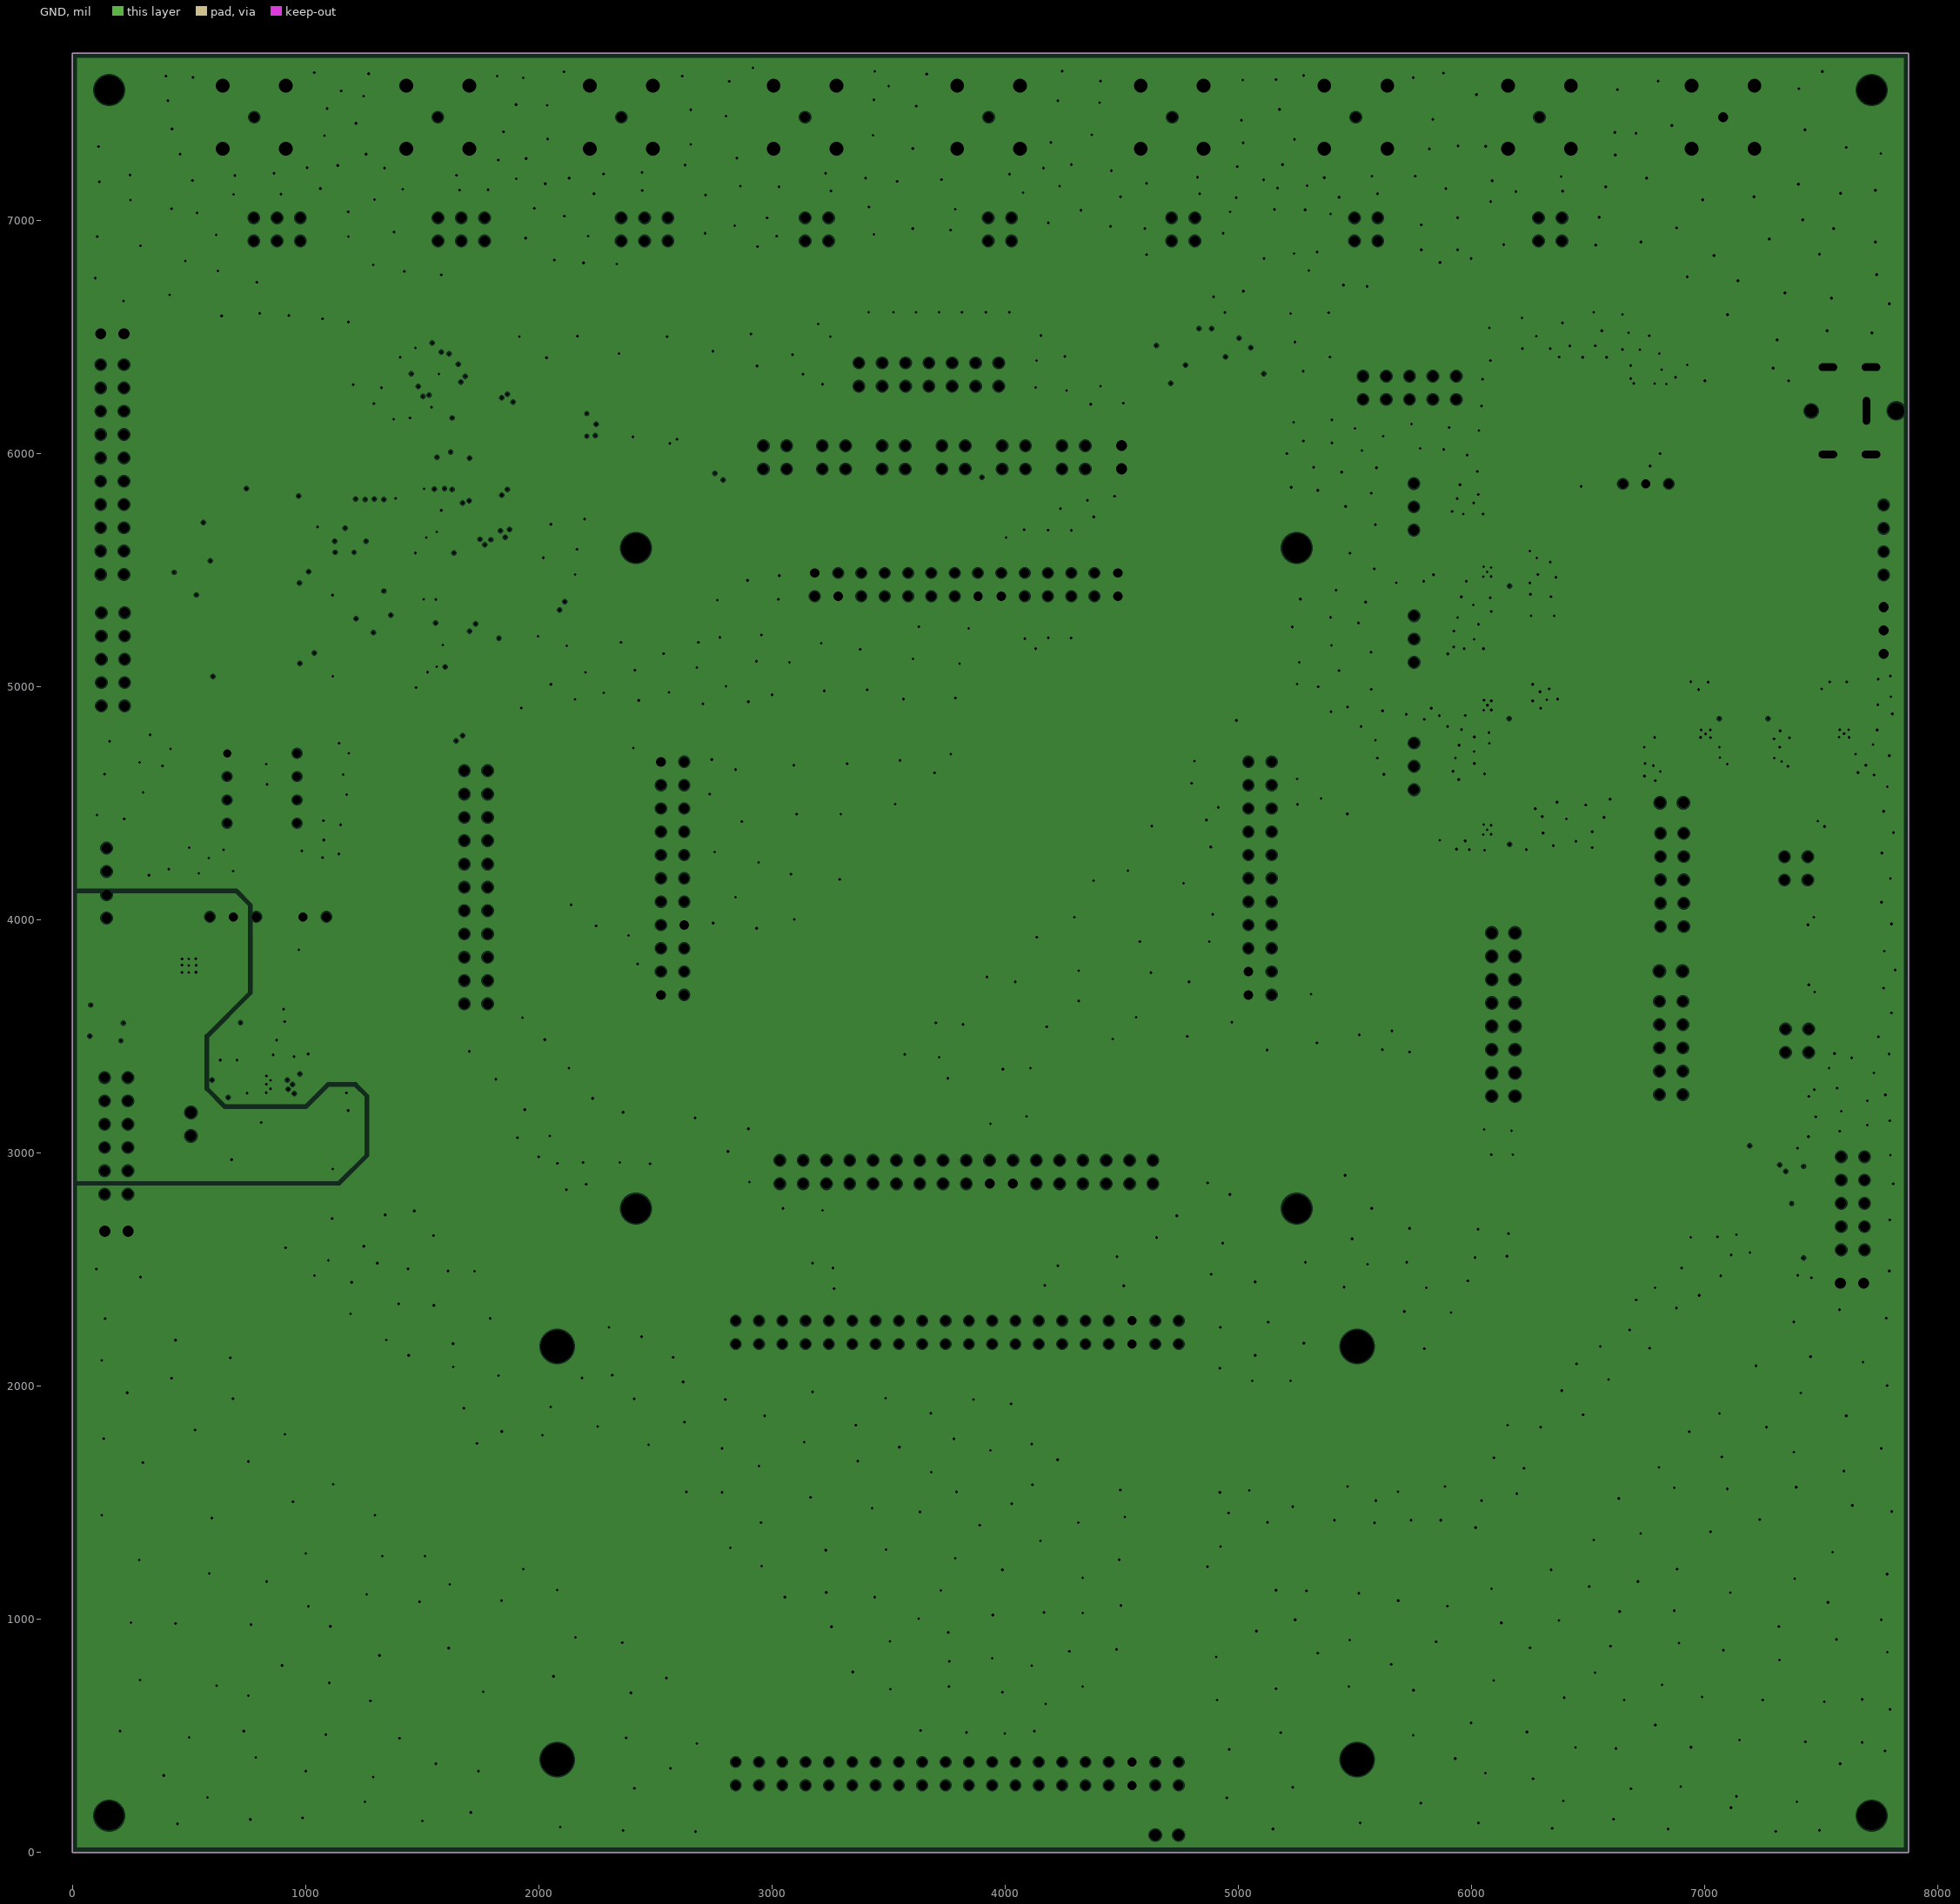
[diagram p0: GND, clearances drawn from the general rule]
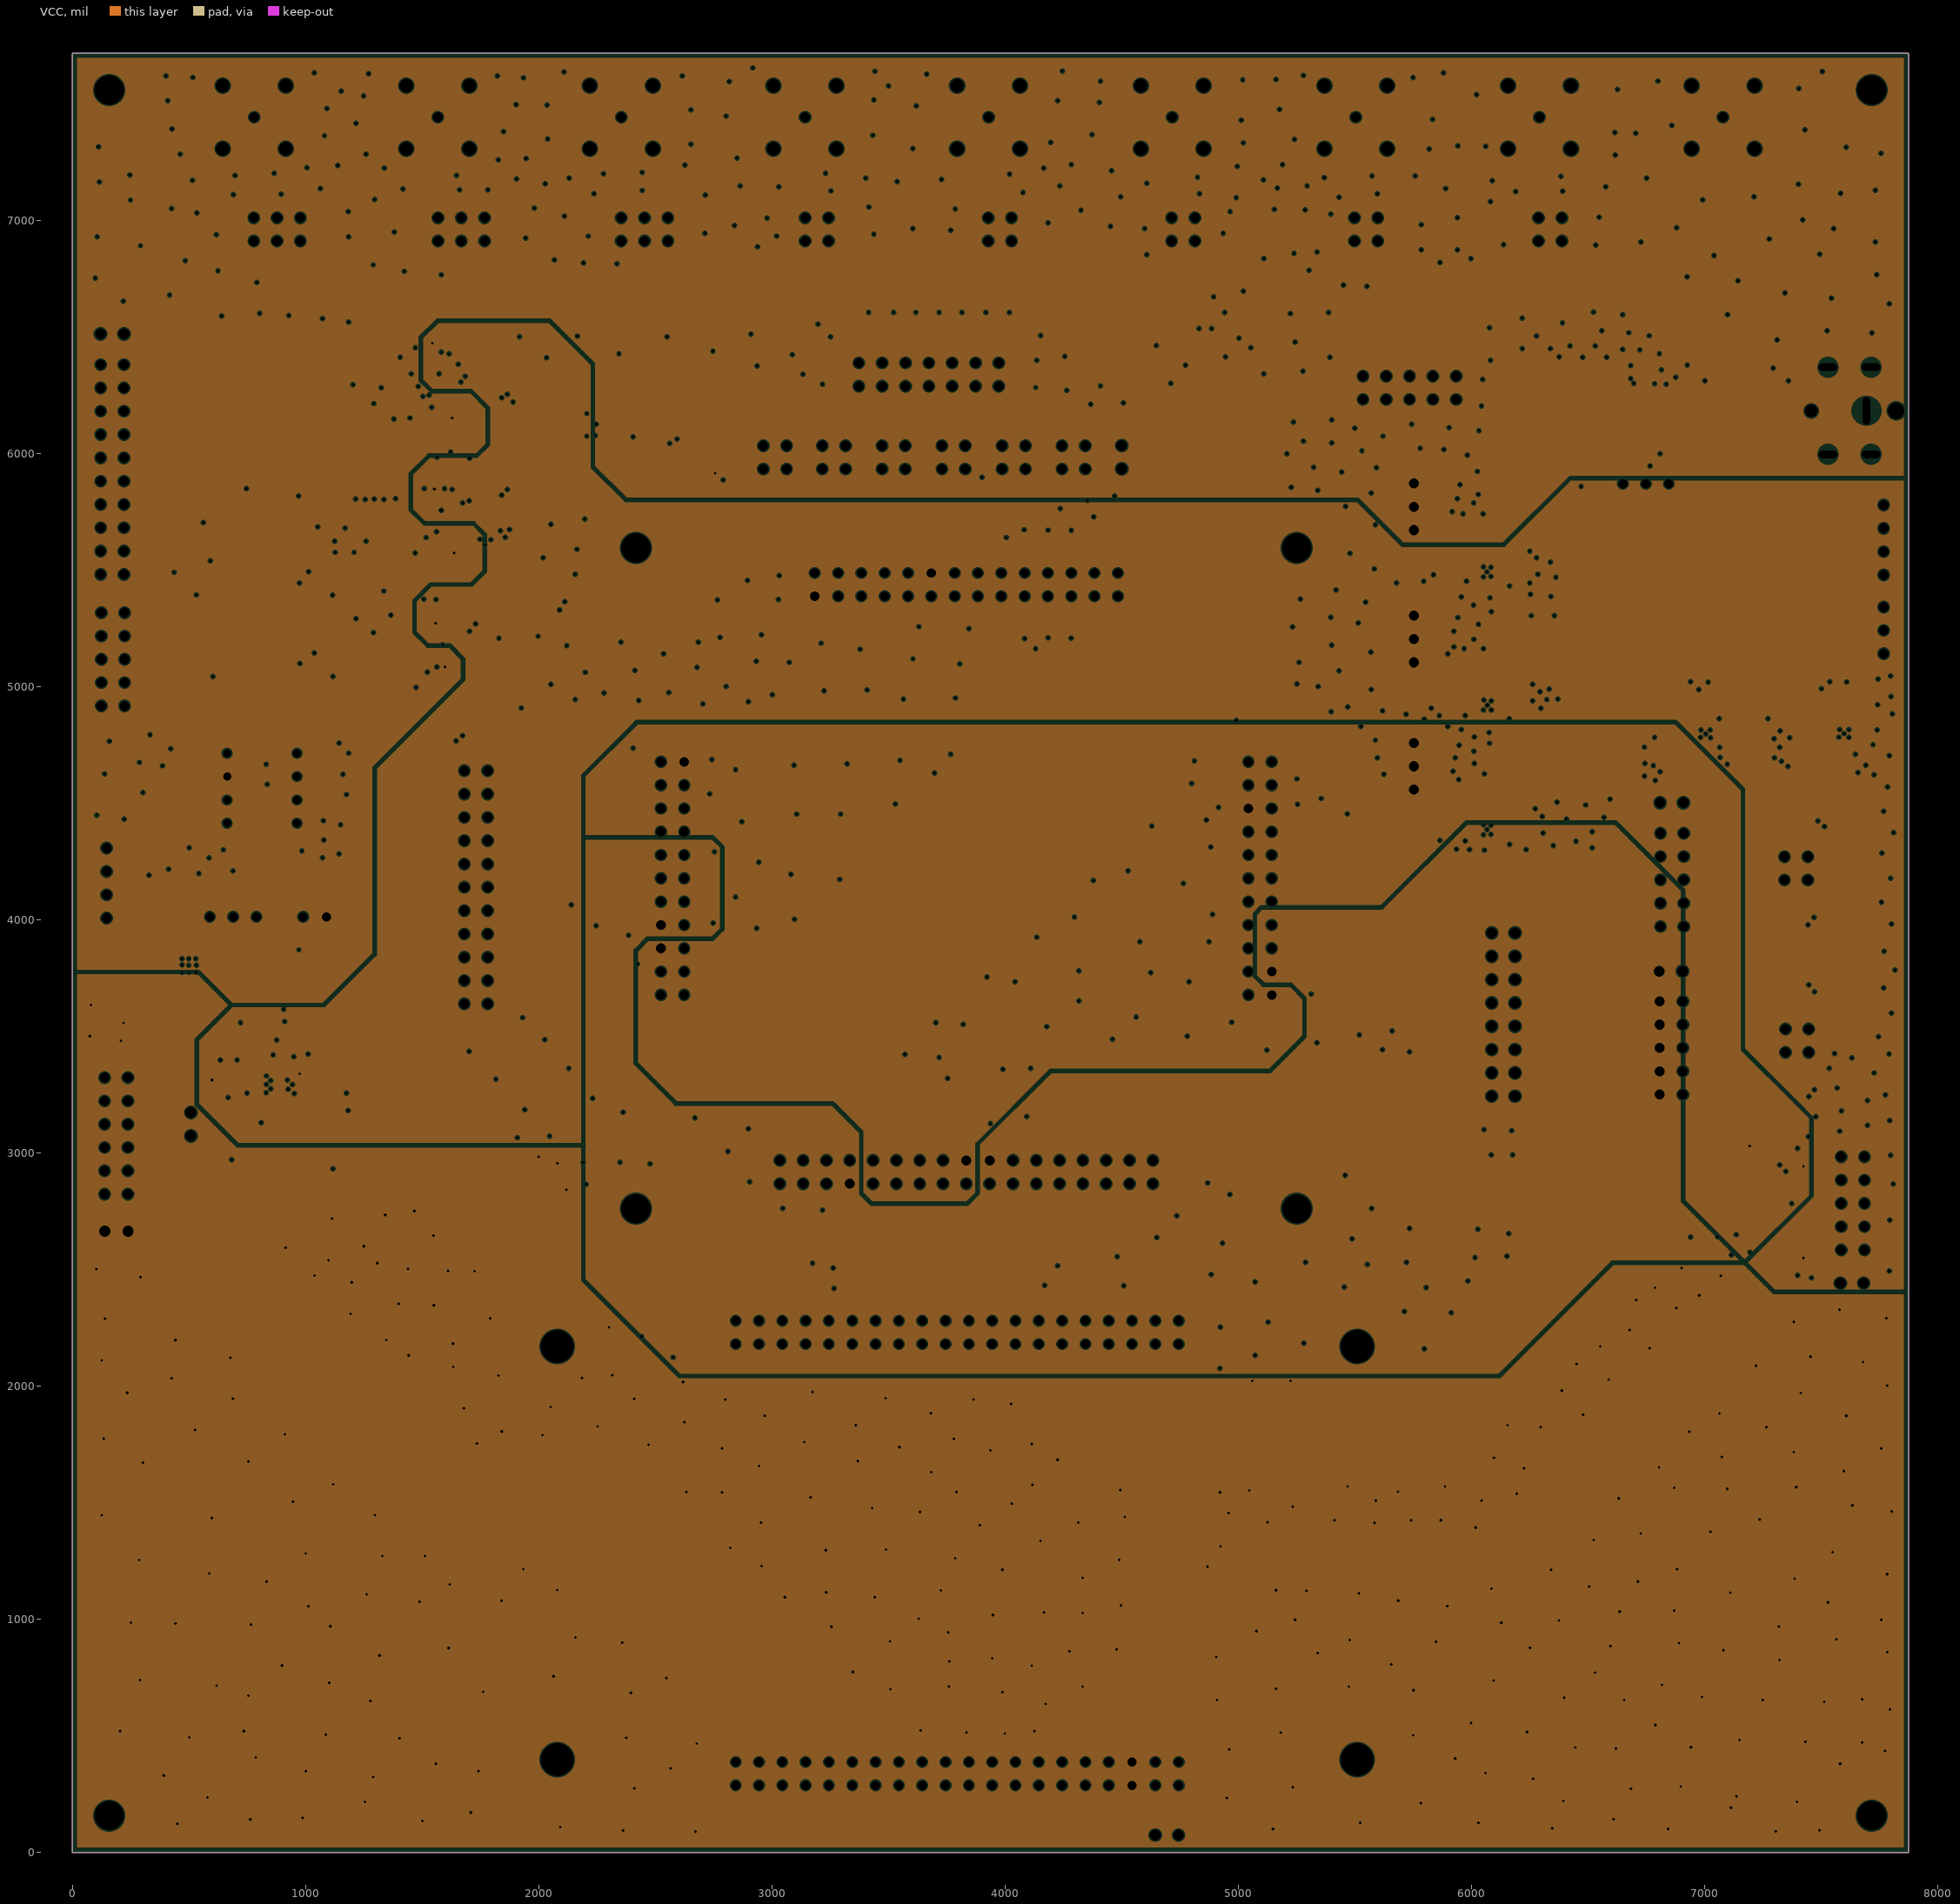
[diagram p1: VCC, clearances drawn from the general rule]
# Altium PCB MISC62793.pcbdoc (part 2 of 6)
## Footprints (in the part's own frame and the unit in brackets; to place one, negate y for a bottom-side part, rotate by r counter-clockwise, add the part's x,y. Pads: shape width x height; smd on the part's side, far side on the other; paste and mask are expansions set on the pad) (continued)
C0402 [mm]
  rect 0.79x0.54 smd paste-100 mask+0.051: 1(-0.545,0) 2(0.545,0)
  silkscreen extent -1.17,-0.5 1.17,0.5
C0603 [mm]
  rect 0.8x0.9 smd: 1(-0.7,0) 2(0.7,0)
  silkscreen extent -1.41,-0.71 1.39,0.72
C0805 [mm]
  rect 1.41x1.35 smd paste-100 mask+0.051: 1(-1,0) 2(1,0)
  silkscreen extent -1.96,-0.9 1.96,0.9
C1206 [mm]
  rect 1.485x1.728 smd paste-100 mask+0.051: 1(-1.593,0) 2(1.593,0)
  silkscreen extent -2.56,-1.09 2.56,1.09
C1210 [mm]
  rect 1.635x2.7 smd paste-100 mask+0.051: 1(-1.517,0) 2(1.517,0)
  silkscreen extent -2.56,-1.58 2.56,1.58
DC-IN-TH_HX-DC007B-2.5 [mm]
  round 1.8 hole 1.8 unplated: 0(-6,0)
  round 2.2 hole 1.4: 1(3.25,0)
  oval 1.4x3.8 hole 0.8 slot 3 at 90 deg: 2(-2.75,0)
  oval 2.8x1.4 hole 0.8 slot 2 at 0 deg: 3(-3.25,4.75) 3(-3.25,-4.75) 3(1.45,4.75) 3(1.45,-4.75)
  silkscreen extent -8.75,-5 4.25,5
DIP-8_L10.1-W6.3-P2.54-LS7.6-BL [mm]
  rect 1.5x1.5 hole 0.9: 1(-3.81,-3.81)
  round 1.5 hole 0.9: 2(-1.27,-3.81) 3(1.27,-3.81) 4(3.81,-3.81) 5(3.81,3.81) 6(1.27,3.81) 7(-1.27,3.81) 8(-3.81,3.81)
  silkscreen extent -5.23,-3.93 5.01,3.18
FILTER-SMD_4P-L7.0-W6.0-TL_SMCM7060 [mm]
  rect 2.5x1.75 smd: 1(-2.75,1.625) 2(-2.75,-1.625) 3(2.75,-1.625) 4(2.75,1.625)
  silkscreen extent -3.94,-3.05 3.94,3.05
HDR-TH_2P-P2.54-V-M [mm]
  rect 2x2 hole 1.2: 1(-1.27,0)
  round 2 hole 1.2: 2(1.27,0)
  silkscreen extent -2.54,-1.27 2.54,1.27
HDR-TH_3P-P2.54-V-M [mm]
  rect 1.7x1.7 hole 1.1: 1(-2.54,0)
  round 1.7 hole 1.1: 2(0,0) 3(2.54,0)
  silkscreen extent -4.02,-1.27 4.02,1.27
HDR-TH_4P-P2.54-V-M [mm]
  rect 1.7x1.7 hole 1.1: 1(-3.81,0)
  round 1.7 hole 1.1: 2(-1.27,0) 3(1.27,0) 4(3.81,0)
  silkscreen extent -5.08,-1.27 5.08,1.27
HDR-TH_4P-P2.54-V-M-R2-C2-S2.54 [mm]
  rect 1.7x1.7 hole 1.1: 1(-1.27,-1.27)
  round 1.7 hole 1.1: 2(-1.27,1.27) 3(1.27,-1.27) 4(1.27,1.27)
  silkscreen extent -2.77,-2.54 2.77,2.54
HDR-TH_6P-P2.54-V-M-R2-C3-S2.54 [mm]
  rect 1.7x1.7 hole 1.1: 1(-2.54,-1.27)
  round 1.7 hole 1.1: 2(-2.54,1.27) 3(0,-1.27) 4(0,1.27) 5(2.54,-1.27) 6(2.54,1.27)
  silkscreen extent -4.04,-2.54 4.04,2.54
HDR-TH_10P-P2.54-V-M-R2-C5-S2.54 [mm]
  rect 1.7x1.7 hole 1.1: 1(-5.08,-1.27)
  round 1.7 hole 1.1: 2(-5.08,1.27) 3(-2.54,-1.27) 4(-2.54,1.27) 5(0,-1.27) 6(0,1.27) 7(2.54,-1.27) 8(2.54,1.27) 9(5.08,-1.27) 10(5.08,1.27)
  silkscreen extent -6.35,-2.54 6.35,2.54
HDR-TH_12P-P2.54-V-M-R2-C6-S2.54 [mm]
  rect 1.7x1.7 hole 1.1: 1(-6.35,-1.27)
  round 1.7 hole 1.1: 2(-6.35,1.27) 3(-3.81,-1.27) 4(-3.81,1.27) 5(-1.27,-1.27) 6(-1.27,1.27) 7(1.27,-1.27) 8(1.27,1.27) 9(3.81,-1.27) 10(3.81,1.27) 11(6.35,-1.27) 12(6.35,1.27)
  silkscreen extent -7.85,-2.54 7.85,2.54
HDR-TH_14P-P2.54-V-M-R2-C7-S2.54 [mm]
  rect 1.7x1.7 hole 1.1: 1(-7.62,-1.27)
  round 1.7 hole 1.1: 2(-7.62,1.27) 3(-5.08,-1.27) 4(-5.08,1.27) 5(-2.54,-1.27) 6(-2.54,1.27) 7(0,-1.27) 8(0,1.27) 9(2.54,-1.27) 10(2.54,1.27) 11(5.08,-1.27) 12(5.08,1.27) 13(7.62,-1.27) 14(7.62,1.27)
  silkscreen extent -9.12,-2.54 9.12,2.54
HDR-TH_16P-P2.54-V-M-R2-C8-S2.54 [mm]
  rect 1.8x1.8 hole 1.2: 1(-8.89,-1.27)
  round 1.8 hole 1.2: 2(-8.89,1.27) 3(-6.35,-1.27) 4(-6.35,1.27) 5(-3.81,-1.27) 6(-3.81,1.27) 7(-1.27,-1.27) 8(-1.27,1.27) 9(1.27,-1.27) 10(1.27,1.27) 11(3.81,-1.27) 12(3.81,1.27) 13(6.35,-1.27) 14(6.35,1.27) 15(8.89,-1.27) 16(8.89,1.27)
  silkscreen extent -10.16,-2.54 10.16,2.54
HDR-TH_20P-P2.54-V-M-R2-C10-S2.54 [mm]
  rect 1.7x1.7 hole 1.1: 1(-11.43,-1.27)
  round 1.7 hole 1.1: 2(-11.43,1.27) 3(-8.89,-1.27) 4(-8.89,1.27) 5(-6.35,-1.27) 6(-6.35,1.27) 7(-3.81,-1.27) 8(-3.81,1.27) 9(-1.27,-1.27) 10(-1.27,1.27) 11(1.27,-1.27) 12(1.27,1.27) 13(3.81,-1.27) 14(3.81,1.27) 15(6.35,-1.27) 16(6.35,1.27) 17(8.89,-1.27) 18(8.89,1.27) 19(11.43,-1.27) 20(11.43,1.27)
  silkscreen extent -12.7,-2.54 12.7,2.54
HDR-TH_22P-P2.54-V-F-R2-C11-S2.54 [mm]
  rect 1.6x1.6 hole 1.05: 1(-12.7,-1.27)
  round 1.6 hole 1.05: 2(-12.7,1.27) 3(-10.16,-1.27) 4(-10.16,1.27) 5(-7.62,-1.27) 6(-7.62,1.27) 7(-5.08,-1.27) 8(-5.08,1.27) 9(-2.54,-1.27) 10(-2.54,1.27) 11(0,-1.27) 12(0,1.27) 13(2.54,-1.27) 14(2.54,1.27) 15(5.08,-1.27) 16(5.08,1.27) 17(7.62,-1.27) 18(7.62,1.27) 19(10.16,-1.27) 20(10.16,1.27) 21(12.7,-1.27) 22(12.7,1.27)
  silkscreen extent -14.22,-2.54 14.22,2.54
HDR-TH_22P-P2.54-V-M-R2-C11-S2.54 [mm]
  rect 1.7x1.7 hole 1.1: 1(-12.7,-1.27)
  round 1.7 hole 1.1: 2(-12.7,1.27) 3(-10.16,-1.27) 4(-10.16,1.27) 5(-7.62,-1.27) 6(-7.62,1.27) 7(-5.08,-1.27) 8(-5.08,1.27) 9(-2.54,-1.27) 10(-2.54,1.27) 11(0,-1.27) 12(0,1.27) 13(2.54,-1.27) 14(2.54,1.27) 15(5.08,-1.27) 16(5.08,1.27) 17(7.62,-1.27) 18(7.62,1.27) 19(10.16,-1.27) 20(10.16,1.27) 21(12.7,-1.27) 22(12.7,1.27)
  silkscreen extent -14.2,-2.54 14.2,2.54
HDR-TH_28P-P2.54-V-F-R2-C14-S2.54-1 [mm]
  rect 1.6x1.6 hole 1.02: 1(-16.51,-1.27)
  round 1.6 hole 1.02: 2(-16.51,1.27) 3(-13.97,-1.27) 4(-13.97,1.27) 5(-11.43,-1.27) 6(-11.43,1.27) 7(-8.89,-1.27) 8(-8.89,1.27) 9(-6.35,-1.27) 10(-6.35,1.27) 11(-3.81,-1.27) 12(-3.81,1.27) 13(-1.27,-1.27) 14(-1.27,1.27) 15(1.27,-1.27) 16(1.27,1.27) 17(3.81,-1.27) 18(3.81,1.27) 19(6.35,-1.27) 20(6.35,1.27) 21(8.89,-1.27) 22(8.89,1.27) 23(11.43,-1.27) 24(11.43,1.27) 25(13.97,-1.27) 26(13.97,1.27) 27(16.51,-1.27) 28(16.51,1.27)
  silkscreen extent -18.03,-2.5 18.03,2.5
HDR-TH_34P-P2.54-V-F-R2-C17-S2.54-1 [mm]
  rect 1.7x1.7 hole 1.1: 1(-20.32,-1.27)
  round 1.7 hole 1.1: 2(-17.78,-1.27) 3(-15.24,-1.27) 4(-12.7,-1.27) 5(-10.16,-1.27) 6(-7.62,-1.27) 7(-5.08,-1.27) 8(-2.54,-1.27) 9(0,-1.27) 10(2.54,-1.27) 11(5.08,-1.27) 12(7.62,-1.27) 13(10.16,-1.27) 14(12.7,-1.27) 15(15.24,-1.27) 16(17.78,-1.27) 17(20.32,-1.27) 18(20.32,1.27) 19(17.78,1.27) 20(15.24,1.27) 21(12.7,1.27) 22(10.16,1.27) 23(7.62,1.27) 24(5.08,1.27) 25(2.54,1.27) 26(0,1.27) 27(-2.54,1.27) 28(-5.08,1.27) 29(-7.62,1.27) 30(-10.16,1.27) 31(-12.7,1.27) 32(-15.24,1.27) 33(-17.78,1.27) 34(-20.32,1.27)
  silkscreen extent -21.84,-2.54 21.84,2.54
HDR-TH_40P-P2.54-V-F-R2-C20-S2.54 [mm]
  rect 1.6x1.6 hole 1: 1(-24.13,-1.27)
  round 1.6 hole 1: 2(-24.13,1.27) 3(-21.59,-1.27) 4(-21.59,1.27) 5(-19.05,-1.27) 6(-19.05,1.27) 7(-16.51,-1.27) 8(-16.51,1.27) 9(-13.97,-1.27) 10(-13.97,1.27) 11(-11.43,-1.27) 12(-11.43,1.27) 13(-8.89,-1.27) 14(-8.89,1.27) 15(-6.35,-1.27) 16(-6.35,1.27) 17(-3.81,-1.27) 18(-3.81,1.27) 19(-1.27,-1.27) 20(-1.27,1.27) 21(1.27,-1.27) 22(1.27,1.27) 23(3.81,-1.27) 24(3.81,1.27) 25(6.35,-1.27) 26(6.35,1.27) 27(8.89,-1.27) 28(8.89,1.27) 29(11.43,-1.27) 30(11.43,1.27) 31(13.97,-1.27) 32(13.97,1.27) 33(16.51,-1.27) 34(16.51,1.27) 35(19.05,-1.27) 36(19.05,1.27) 37(21.59,-1.27) 38(21.59,1.27) 39(24.13,-1.27) 40(24.13,1.27)
  silkscreen extent -25.53,-2.54 25.53,2.54
IND-SMD_L7.3-W6.8 [mm]
  rect 2.35x3.5 smd: 1(-3,0) 2(3,0)
  silkscreen extent -3.5,-3.3 3.5,3.3
LED_0805 [mm]
  rect 1x1.25 smd paste+0 mask+0.051: 1(-1.15,0.005) 2(1.05,0.005)
  silkscreen extent -2.15,-0.94 1.93,0.97
MSOP-8_L3.0-W3.0-P0.65-LS5.0-TL [mil]
  oval 66.61x14.33 smd: 1(-84.49,38.39) 2(-84.49,12.79) 3(-84.49,-12.8) 4(-84.49,-38.39) 5(84.49,-38.39) 6(84.49,-12.8) 7(84.49,12.79) 8(84.49,38.39)
  silkscreen extent -90,-65 68,69
PWRM-TH_A05XXS-1WR3 [mm]
  round 1.6 hole 1: 1(-6.35,0) 2(-3.81,0) 4(1.27,0) 5(3.81,0) 6(6.35,0)
  silkscreen extent -8.56,-5.05 11.1,2.05
R0603 [mil]
  rect 31.75x34.02 smd paste-3937.01 mask+2: 1(-29.66,0) 2(29.66,0)
  silkscreen extent -55,-26 55,26
R0805 [mm]
  rect 1.133x1.377 smd paste-100 mask+0.051: 1(-1,0) 2(1,0)
  silkscreen extent -1.76,-0.92 1.76,0.92
R1206 [mil]
  rect 47.54x66.97 smd paste-3937.01 mask+2: 1(-58.22,0) 2(58.22,0)
  silkscreen extent -91,-42 91,42
RES-ADJ-SMD_3P-L4.5-W4.5-P2.30-BL-FS [mm]
  rect 2x1.3 smd: 1(-2,-1.15) 3(-2,1.15)
  rect 2x2 smd: 2(2,0)
  silkscreen extent -3.28,-2.78 2.25,2.25
RES-ADJ-SMD_3P-L6.0-W4.3-P5.00-BL [mm]
  rect 1.4x2 smd: 1(-2.5,-2.65) 2(0,2.65) 3(2.5,-2.65)
  silkscreen extent -3,-2.15 3,2.15
SMA_L4.2-W2.7-LS5.0-BI [mm]
  rect 2x1.8 smd: 1(-2,0) 2(2,0)
  silkscreen extent -2.3,-1.4 2.3,1.4
SMB_L4.6-W3.6-LS5.3-RD [mil]
  rect 80.61x86.31 smd: 1(-92.94,0) 2(92.94,0)
  silkscreen extent -123,-77 108,77
SOIC-8_L4.9-W3.9-P1.27-LS6.0-BL [mm]
  oval 0.588x2.045 smd: 1(-1.905,-2.772) 2(-0.635,-2.772) 3(0.635,-2.772) 4(1.905,-2.772) 5(1.905,2.772) 6(0.635,2.772) 7(-0.635,2.772) 8(-1.905,2.772)
  silkscreen extent -2.8,-2.92 2.53,1.52
SW-TH_K3-1204D [mm]
  round 1.5 hole 1: 1(-2.5,0) 2(0,0) 3(2.5,0)
  silkscreen extent -5,-1.25 5,1.25
TSSOP-20_L6.5-W4.4-P0.65-LS6.4-BL [mil]
  oval 14.33x68.58 smd: 1(-115.16,-113.03) 2(-89.57,-113.03) 3(-63.98,-113.03) 4(-38.39,-113.03) 5(-12.79,-113.03) 6(12.8,-113.03) 7(38.39,-113.03) 8(63.98,-113.03) 9(89.57,-113.03) 10(115.16,-113.03) 11(115.16,113.03) 12(89.57,113.03) 13(63.98,113.03) 14(38.39,113.03) 15(12.8,113.03) 16(-12.79,113.03) 17(-38.39,113.03) 18(-63.98,113.03) 19(-89.57,113.03) 20(-115.16,113.03)
  silkscreen extent -146,-119 131,70
VQFN-10_L2.0-W2.0-P0.45-TL [mm]
  round 0.6 smd: 1(-0.915,0.9) 4(-0.905,-0.9) 7(0.915,-0.9) 10(0.915,0.9)
  rect 0.6x0.25 smd paste+0 mask+0.05: 2(-0.905,0.225) 3(-0.905,-0.225) 8(0.905,-0.225) 9(0.905,0.225)
  rect 0.3x2.4 smd paste+0 mask+0.05: 5(-0.235,0) 6(0.265,0)
  Top Layer region: -0.865,1.2 -0.865,0.9 -1.215,0.9 -1.215,0.6 -0.865,0.6 -0.615,0.6 -0.615,0.6 -0.615,0.9 -0.615,0.9 -0.615,1.2 -0.865,1.2
  Top Layer region: -0.855,-1.2 -0.855,-0.9 -1.205,-0.9 -1.205,-0.6 -0.855,-0.6 -0.605,-0.6 -0.605,-0.6 -0.605,-0.9 -0.605,-0.9 -0.605,-1.2 -0.855,-1.2
  Top Layer region: 0.865,-1.2 0.865,-0.9 1.215,-0.9 1.215,-0.6 0.865,-0.6 0.615,-0.6 0.615,-0.6 0.615,-0.9 0.615,-0.9 0.615,-1.2 0.865,-1.2
  Top Layer region: 0.865,1.2 0.865,0.9 1.215,0.9 1.215,0.6 0.865,0.6 0.615,0.6 0.615,0.6 0.615,0.9 0.615,0.9 0.615,1.2 0.865,1.2
  silkscreen extent -1.85,-1.28 1.34,1.36
VSON-8_L3.0-W3.0-P0.65-TL-EP [mm]
  rect 0.85x0.34 smd: 1(-1.476,0.975) 2(-1.476,0.325) 3(-1.476,-0.325) 4(-1.476,-0.975) 5(1.476,-0.975) 6(1.476,-0.325) 7(1.476,0.325) 8(1.476,0.975)
  rect 1.52x1.78 smd: 9(0,0)
  Top Layer region: -0.76,0.89 -0.47,0.89 -0.47,1.71 -0.18,1.71 -0.18,0.88 0.18,0.88 0.18,1.71 0.47,1.71 0.47,0.88 0.76,0.88 0.76,-0.89 0.47,-0.89 0.47,-1.71 0.18,-1.71 0.18,-0.89 -0.18,-0.89 -0.18,-1.71 -0.47,-1.71 -0.47,-0.89 -0.76,-0.89 -0.76,0.89 -0.76,0.89
  silkscreen extent -1.96,-1.52 1.52,1.58
VSON-10_L3.0-W3.0-P0.50-TL-EP-3 [mm]
  rect 0.8x0.25 smd paste+0 mask+0.05: 1(-1.4,1) 2(-1.4,0.5) 3(-1.4,0) 4(-1.4,-0.5) 5(-1.4,-1) 6(1.4,-1) 7(1.4,-0.5) 8(1.4,0) 9(1.4,0.5) 10(1.4,1)
  rect 0.25x0.8 smd paste+0 mask+0.05: 11(0,0)
  Top Layer region: -0.295,1.275 -0.295,1.5 -0.525,1.5 -0.525,-1.5 -0.295,-1.5 -0.295,-1.275 0.295,-1.275 0.295,-1.5 0.525,-1.5 0.525,-1.275 0.525,-1.275 0.525,1.275 0.525,1.275 0.525,1.5 0.295,1.5 0.295,1.275 -0.295,1.275
  silkscreen extent -2.26,-1.5 1.5,1.5
VSSOP-10_L3.0-W3.0-P0.50-LS4.9-BL [mm]
  rect 0.3x1.3 smd paste+0 mask+0.015: 1(-1,-2.35) 2(-0.5,-2.35) 3(0,-2.35) 4(0.5,-2.35) 5(1,-2.35)
  rect 0.3x1.3 smd: 6(1,2.35) 7(0.5,2.35) 8(0,2.35) 9(-0.5,2.35) 10(-1,2.35)
  silkscreen extent -1.62,-2.08 1.52,1.54
WQFN-16_L3.0-W3.0-P0.50-TL-EP0.8 [mm]
  rect 0.85x0.28 smd paste+0 mask+0.05: 1(-1.5,0.75) 2(-1.5,0.25) 3(-1.5,-0.25) 4(-1.5,-0.75) 9(1.5,-0.75) 10(1.5,-0.25) 11(1.5,0.25) 12(1.5,0.75)
  rect 0.28x0.85 smd paste+0 mask+0.05: 5(-0.75,-1.5) 6(-0.25,-1.5) 7(0.25,-1.5) 8(0.75,-1.5) 13(0.75,1.5) 14(0.25,1.5) 15(-0.25,1.5) 16(-0.75,1.5)
  rect 0.8x0.8 smd paste+0 mask+0.05: 17(0,0)
  silkscreen extent -2.39,-1.5 1.5,1.5